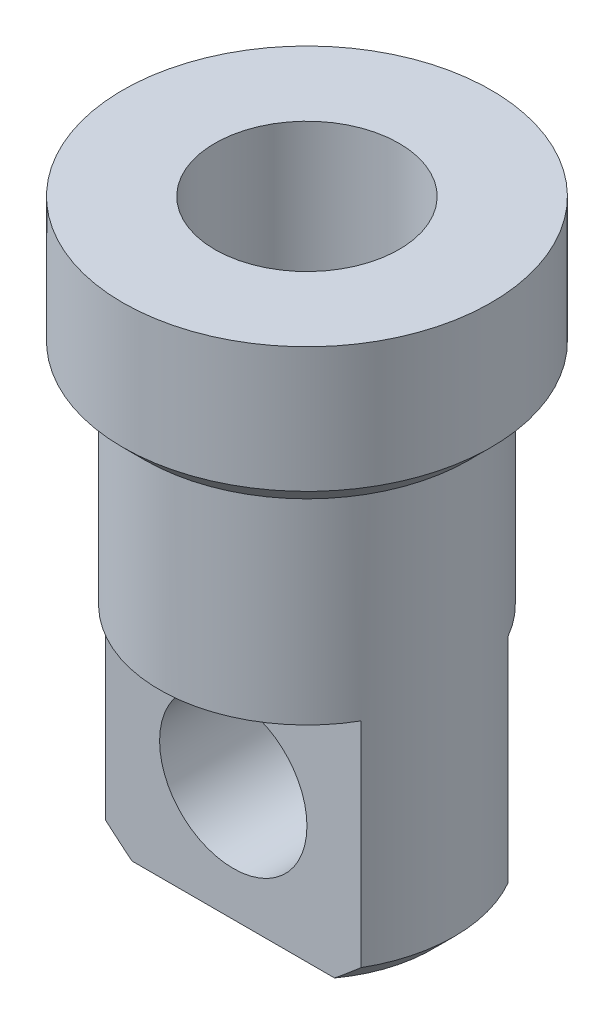
from build123d import *

# Parameters (mm, degrees)
SKETCH1_R             = 2
BOSS_EXTRUDE1_DEPTH   = 6
SKETCH2_R             = 2.5
BOSS_EXTRUDE2_DEPTH   = 2
M3_TAPPED_HOLE1_D     = 2.5
M3_TAPPED_HOLE1_DEPTH = 4.5
M3_TAPPED_HOLE1_TIP   = 0.751075774
CHAMFER1_SIZE         = 0.3
SKETCH6_R             = 1
CUT_EXTRUDE1_DEPTH    = 5
SKETCH7_W             = 3
SKETCH7_H             = 3.2
CUT_EXTRUDE2_DEPTH    = 5


with BuildPart() as part:
    # Sketch1 → Boss-Extrude1 (new body)
    with BuildSketch(Plane(origin=(0, 0, 0), x_dir=(1, 0, 0), z_dir=(0, 1, 0))):
        with Locations(Location((0, 0, 0), (0, 0, 270))):
            Circle(SKETCH1_R)
    extrude(amount=BOSS_EXTRUDE1_DEPTH)

    # Sketch2 → Boss-Extrude2 (add)
    with BuildSketch(Plane(origin=(0, 6, 0), x_dir=(1, 0, 0), z_dir=(0, 1, 0))):
        with Locations(Location((0, 0, 0), (0, 0, 270))):
            Circle(SKETCH2_R)
    extrude(amount=BOSS_EXTRUDE2_DEPTH)

    # M3 Tapped Hole1
    with Locations(Plane(origin=(0, 8, 0), x_dir=(1, 0, 0), z_dir=(0, 1, 0))):
        with Locations((0, 0)):
            Hole(M3_TAPPED_HOLE1_D / 2, depth=M3_TAPPED_HOLE1_DEPTH)
            with Locations((0, 0, -(M3_TAPPED_HOLE1_DEPTH + M3_TAPPED_HOLE1_TIP / 2))):  # 118° drill point
                Cone(0, M3_TAPPED_HOLE1_D / 2, M3_TAPPED_HOLE1_TIP, mode=Mode.SUBTRACT)

    # Chamfer1
    chamfer1_edges = [part.edges().sort_by_distance(p)[0] for p in [
        (0, 0, -2),
        (0, 6, -2.5),
    ]]
    chamfer(chamfer1_edges, length=CHAMFER1_SIZE)

    # Sketch6 → Cut-Extrude1 (cut, symmetric)
    with BuildSketch(Plane.XY):
        with Locations(Location((0, 1.6, 0), (0, 0, 90.00000001))):
            Circle(SKETCH6_R)
    extrude(amount=CUT_EXTRUDE1_DEPTH, both=True, mode=Mode.SUBTRACT)

    # Sketch7 → Cut-Extrude2 (cut, symmetric)
    with BuildSketch(Plane(origin=(0, 0, 0), x_dir=(0, 0, -1), z_dir=(1, 0, 0))):
        with Locations((2.5, 1.6)):
            Rectangle(SKETCH7_W, SKETCH7_H)
        with Locations((-2.5, 1.6)):
            Rectangle(SKETCH7_W, SKETCH7_H)
    extrude(amount=CUT_EXTRUDE2_DEPTH, both=True, mode=Mode.SUBTRACT)


solid = part.part
